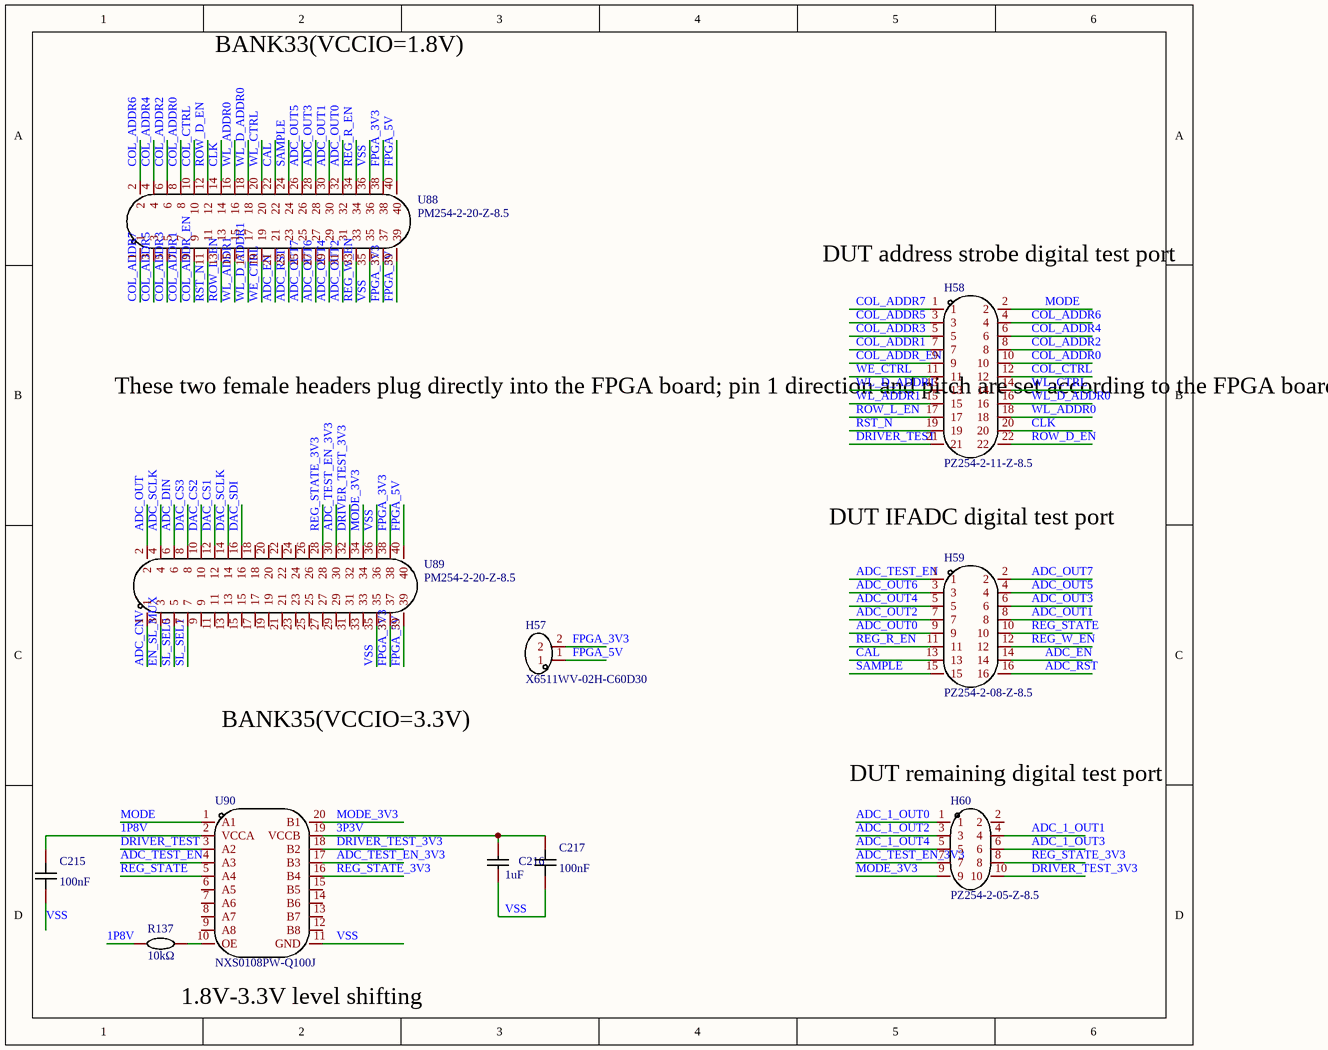
[diagram p0: MISC62793-8.schdoc]
# Altium project MISC62793-14.PrjPcb (part 4 of 4)

## Nets that join several sheets
VSS: MISC62793-2 (66 pins), MISC62793-4 (85 pins), MISC62793-6 (20 pins), MISC62793-8 (8 pins)
1P8V: MISC62793-2 (8 pins), MISC62793-6 (5 pins), MISC62793-8 (C215.2 R137.1 U90.2)
3P3V: MISC62793-2 (8 pins), MISC62793-4 (12 pins), MISC62793-6 (U86.17 U86.28), MISC62793-8 (C216.2 C217.2 U90.19)
ADC_1_OUT0: MISC62793-6 (U83.22), MISC62793-8 (H60.1)
ADC_1_OUT1: MISC62793-6 (U83.14), MISC62793-8 (H60.4)
ADC_1_OUT2: MISC62793-6 (U83.21), MISC62793-8 (H60.3)
ADC_1_OUT3: MISC62793-6 (U83.15), MISC62793-8 (H60.6)
ADC_1_OUT4: MISC62793-6 (U83.20), MISC62793-8 (H60.5)
ADC_CNV: MISC62793-4 (H56.2 U71.6), MISC62793-8 (U89.1)
ADC_DIN: MISC62793-4 (H56.5 U71.9), MISC62793-8 (U89.6)
ADC_EN: MISC62793-6 (U83.23), MISC62793-8 (H59.14 U88.21)
ADC_OUT: MISC62793-4 (H56.1 U71.7), MISC62793-8 (U89.2)
ADC_OUT0: MISC62793-6 (U85.8), MISC62793-8 (H59.9 U88.32)
ADC_OUT1: MISC62793-6 (U85.9), MISC62793-8 (H59.8 U88.30)
ADC_OUT2: MISC62793-6 (U85.10), MISC62793-8 (H59.7 U88.31)
ADC_OUT3: MISC62793-6 (U85.11), MISC62793-8 (H59.6 U88.28)
ADC_OUT4: MISC62793-6 (U85.12), MISC62793-8 (H59.5 U88.29)
ADC_OUT5: MISC62793-6 (U85.13), MISC62793-8 (H59.4 U88.26)
ADC_OUT6: MISC62793-6 (U85.14), MISC62793-8 (H59.3 U88.27)
ADC_OUT7: MISC62793-6 (U85.15), MISC62793-8 (H59.2 U88.25)
ADC_RST: MISC62793-6 (U83.13), MISC62793-8 (H59.16 U88.23)
ADC_SCLK: MISC62793-4 (H56.3 U71.8), MISC62793-8 (U89.4)
ADC_TEST_EN: MISC62793-6 (U85.16), MISC62793-8 (H59.1 U90.4)
AVDD: MISC62793-2 (6 pins), MISC62793-6 (U86.3 U86.13)
BL_TEST: MISC62793-4 (H53.10), MISC62793-6 (U85.20)
BNC_AVDD: MISC62793-2 (C152.2 H29.4), MISC62793-4 (H39.1)
BNC_DVDD: MISC62793-2 (C150.2 H28.4), MISC62793-4 (H38.1)
CAL: MISC62793-6 (U83.24), MISC62793-8 (H59.13 U88.22)
CD: MISC62793-4 (H34.3), MISC62793-6 (U83.33)
CLK: MISC62793-6 (U83.30), MISC62793-8 (H58.20 U88.14)
COL_ADDR0: MISC62793-6 (U84.12), MISC62793-8 (H58.10 U88.8)
COL_ADDR1: MISC62793-6 (U84.11), MISC62793-8 (H58.7 U88.7)
COL_ADDR2: MISC62793-6 (U84.10), MISC62793-8 (H58.8 U88.6)
COL_ADDR3: MISC62793-6 (U84.9), MISC62793-8 (H58.5 U88.5)
COL_ADDR4: MISC62793-6 (U84.8), MISC62793-8 (H58.6 U88.4)
COL_ADDR5: MISC62793-6 (U84.7), MISC62793-8 (H58.3 U88.3)
COL_ADDR6: MISC62793-6 (U84.6), MISC62793-8 (H58.4 U88.2)
COL_ADDR7: MISC62793-6 (U84.5), MISC62793-8 (H58.1 U88.1)
COL_ADDR_EN: MISC62793-6 (U84.13), MISC62793-8 (H58.9 U88.9)
COL_CTRL: MISC62793-6 (U84.14), MISC62793-8 (H58.12 U88.10)
DAC_CS1: MISC62793-4 (H56.9 U60.12), MISC62793-8 (U89.12)
DAC_CS2: MISC62793-4 (H56.10 U61.12), MISC62793-8 (U89.10)
DAC_CS3: MISC62793-4 (H56.7 U62.12), MISC62793-8 (U89.8)
DAC_SCLK: MISC62793-4 (H56.12 U60.13 U61.13 U62.13), MISC62793-8 (U89.14)
DAC_SDI: MISC62793-4 (H56.11 U60.14 U61.14 U62.14), MISC62793-8 (U89.16)
DAC_VDD: MISC62793-2 (8 pins), MISC62793-4 (16 pins)
DRIVER_TEST: MISC62793-6 (U83.16), MISC62793-8 (H58.21 U90.3)
DVDD: MISC62793-2 (6 pins), MISC62793-6 (U83.4 U83.25 U84.15 U85.3)
EGD: MISC62793-4 (H34.1), MISC62793-6 (U84.20)
EGG: MISC62793-4 (H33.1), MISC62793-6 (U84.19)
EGS: MISC62793-4 (H35.1), MISC62793-6 (U84.18)
EN_SL_MUX: MISC62793-4 (H56.4 MUX1.5), MISC62793-8 (U89.3)
MODE: MISC62793-6 (U84.4), MISC62793-8 (H58.2 U90.1)
NCSVB: MISC62793-4 (H52.7 U60.10), MISC62793-6 (C208.1 U86.5)
NEG_5V: MISC62793-4 (H52.20 R116.2 U65.6), MISC62793-6 (U86.15)
NG: MISC62793-4 (H33.3), MISC62793-6 (U83.3)
NS: MISC62793-4 (H35.3), MISC62793-6 (U83.32)
OTA_TEST_OUT: MISC62793-4 (H53.9), MISC62793-6 (U83.19)
OTA_TEST_VB: MISC62793-4 (H52.16 U60.11), MISC62793-6 (U83.17)
PG: MISC62793-4 (H32.1), MISC62793-6 (U83.2)
PS: MISC62793-4 (H36.1), MISC62793-6 (U83.34)
REG_R_EN: MISC62793-6 (U85.6), MISC62793-8 (H59.11 U88.34)
REG_STATE: MISC62793-6 (U85.7), MISC62793-8 (H59.10 U90.5)
REG_W_EN: MISC62793-6 (U85.5), MISC62793-8 (H59.12 U88.33)
ROW_D_EN: MISC62793-6 (U83.31), MISC62793-8 (H58.22 U88.12)
ROW_L_EN: MISC62793-6 (U83.6), MISC62793-8 (H58.17 U88.13)
RST_N: MISC62793-6 (U83.5), MISC62793-8 (H58.19 U88.11)
SAMPLE: MISC62793-6 (U83.12), MISC62793-8 (H59.15 U88.24)
SL_SEL0: MISC62793-4 (H56.6 MUX1.1), MISC62793-8 (U89.5)
SL_SEL1: MISC62793-4 (H56.8 MUX1.10), MISC62793-8 (U89.7)
SL_TEST: MISC62793-4 (H53.8), MISC62793-6 (U85.21)
V_ADC_TEST: MISC62793-4 (5 pins), MISC62793-6 (U86.4)
VB_CLAMP: MISC62793-4 (H52.9 U60.2), MISC62793-6 (C202.1 U86.11)
VB_CM: MISC62793-4 (H52.11 U60.4), MISC62793-6 (C204.1 U86.9)
VB_CMP: MISC62793-4 (H52.5 U60.8), MISC62793-6 (C206.1 U86.7)
VBL1: MISC62793-4 (H42.2 H42.4), MISC62793-6 (U86.22)
VBL2: MISC62793-4 (H43.2 H43.4), MISC62793-6 (U86.21)
VBL_DARK: MISC62793-4 (H45.2 H45.4), MISC62793-6 (U86.18)
VCB: MISC62793-4 (H52.12 U60.5), MISC62793-6 (C205.1 U86.8)
VCLAMP: MISC62793-4 (H52.10 U60.3), MISC62793-6 (C203.1 U86.10)
VMH: MISC62793-4 (H52.14 R112.2 U64.6), MISC62793-6 (U84.3)
VML: MISC62793-4 (H52.18 R114.2 U66.6), MISC62793-6 (U86.16)
VSL: MISC62793-4 (MUX1.8), MISC62793-6 (U86.20)
VTH_CMP: MISC62793-4 (H52.6 U60.9), MISC62793-6 (C207.1 U86.6)
VWL1: MISC62793-4 (H40.2 H40.4), MISC62793-6 (U86.25)
VWL2: MISC62793-4 (H41.2 H41.4), MISC62793-6 (U86.24)
VWL_DARK: MISC62793-4 (H44.2 H44.4), MISC62793-6 (U86.19)
WE_CTRL: MISC62793-6 (U83.9), MISC62793-8 (H58.11 U88.19)
WELL: MISC62793-4 (H37.1), MISC62793-6 (U83.1)
WL_ADDR0: MISC62793-6 (U83.29), MISC62793-8 (H58.18 U88.16)
WL_ADDR1: MISC62793-6 (U83.7), MISC62793-8 (H58.15 U88.15)
WL_CTRL: MISC62793-6 (U83.27), MISC62793-8 (H58.14 U88.20)
WL_D_ADDR0: MISC62793-6 (U83.28), MISC62793-8 (H58.16 U88.18)
WL_D_ADDR1: MISC62793-6 (U83.8), MISC62793-8 (H58.13 U88.17)
WL_TEST: MISC62793-4 (H53.7), MISC62793-6 (U85.19)